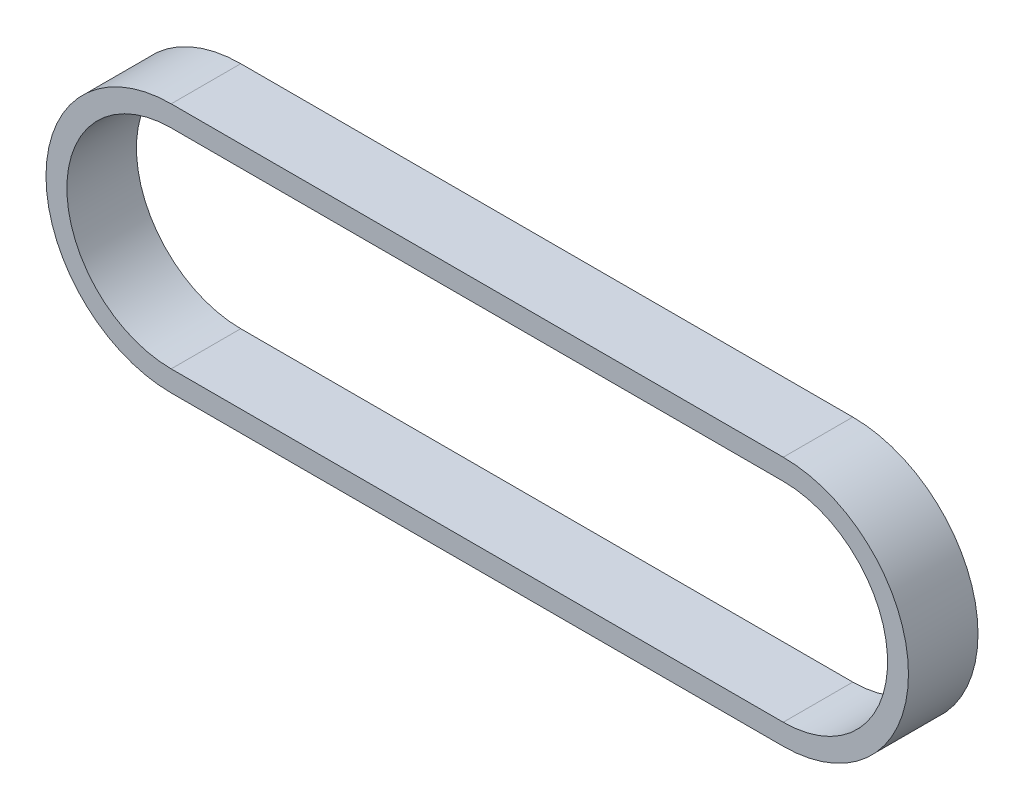
from build123d import *

# Parameters (mm, degrees)
BOSS_EXTRUDE1_DEPTH = 10
SHELL1_T            = -3


with BuildPart() as part:
    # Sketch2 → Boss-Extrude1 (new body)
    with BuildSketch(Plane.XY):
        with BuildLine():
            Line((0, 18), (-88, 18))
            ThreePointArc((-88, 18), (-106, 0), (-88, -18))
            Line((-88, -18), (0, -18))
            ThreePointArc((0, -18), (18, 0), (0, 18))
        make_face()
    extrude(amount=BOSS_EXTRUDE1_DEPTH)

    # Shell1
    shell1_openings = [part.faces().sort_by_distance(p)[0] for p in [
        (-44, 0, 10),
        (-44, 0, 0),
    ]]
    offset(amount=SHELL1_T, openings=shell1_openings, kind=Kind.INTERSECTION)


solid = part.part
